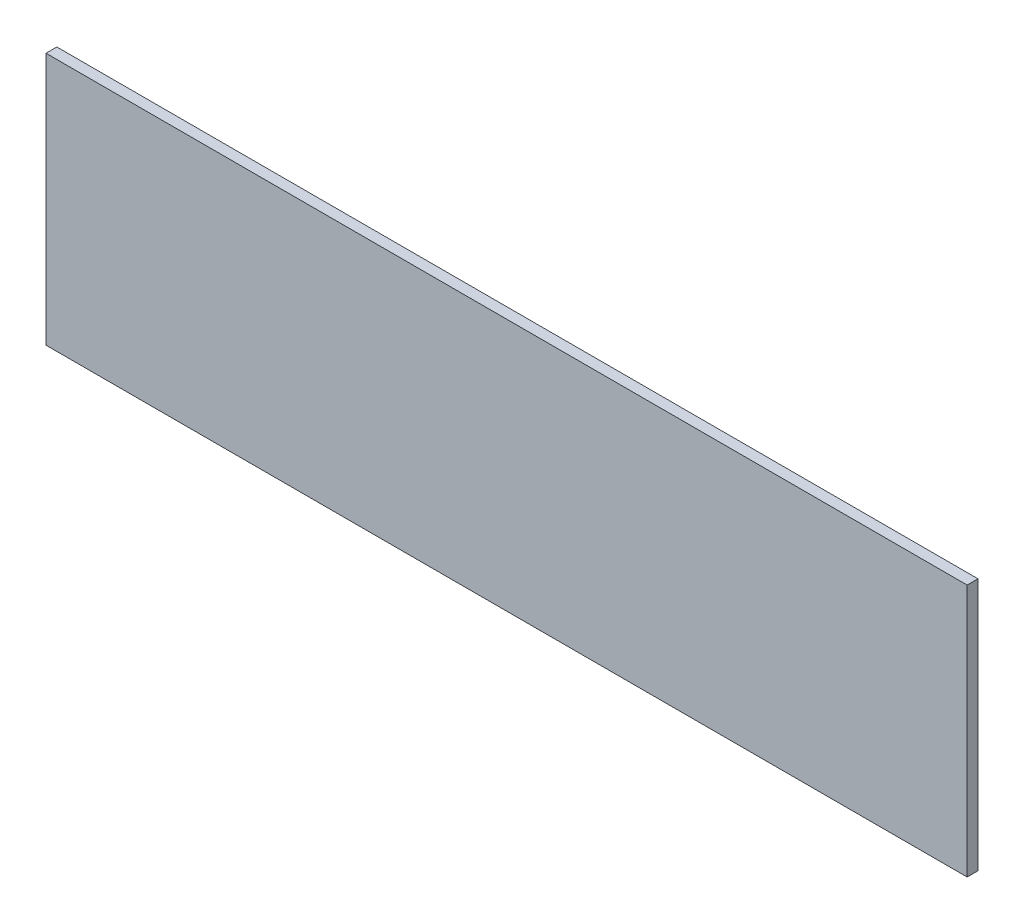
SolidWorks part; units mm, degrees
ref_plane "前视基准面" through (0, 0, 0) normal (0, 0, 1) x (1, 0, 0)
ref_plane "上视基准面" through (0, 0, 0) normal (0, 1, 0) x (1, 0, 0)
ref_plane "右视基准面" through (0, 0, 0) normal (1, 0, 0) x (0, 0, -1)
sketch "草图1" plane through (0, 0, 0) normal (0, 0, 1) x (1, 0, 0)
  line L0 (0, 0) -> (255, 0)
  line L1 (255, 0) -> (255, 70)
  line L2 (255, 70) -> (0, 70)
  line L3 (0, 70) -> (0, 0)
extrude "凸台-拉伸1" add sketch "草图1" along normal blind 3
